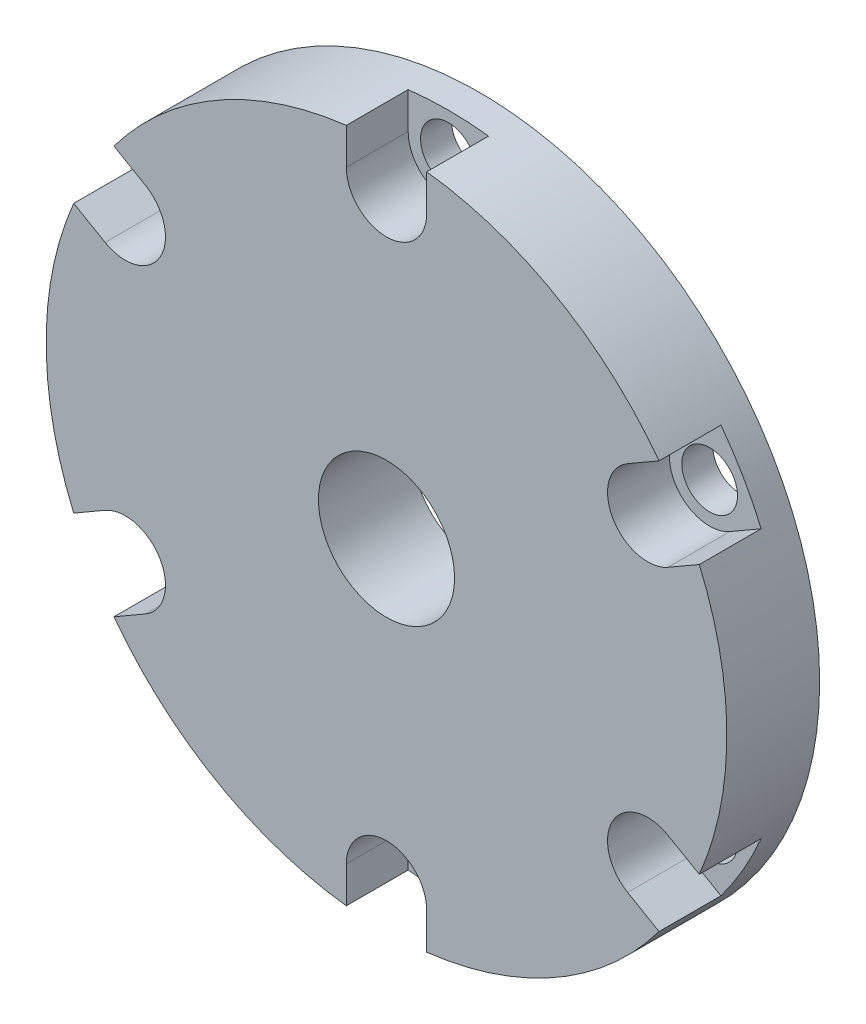
from build123d import *

# Parameters (mm, degrees)
SKETCH1_R           = 110
SKETCH1_R_2         = 9
SKETCH1_R_3         = 22
BOSS_EXTRUDE1_DEPTH = 30
CUT_EXTRUDE1_DEPTH  = 20


with BuildPart() as part:
    # Sketch1 → Boss-Extrude1 (new body)
    with BuildSketch(Plane.XY):
        Circle(SKETCH1_R)
        with Locations((0, 97.5)):
            Circle(SKETCH1_R_2, mode=Mode.SUBTRACT)
        with Locations((84.437476869, 48.75)):
            Circle(SKETCH1_R_2, mode=Mode.SUBTRACT)
        with Locations((84.437476869, -48.75)):
            Circle(SKETCH1_R_2, mode=Mode.SUBTRACT)
        with Locations((0, -97.5)):
            Circle(SKETCH1_R_2, mode=Mode.SUBTRACT)
        with Locations((-84.437476869, -48.75)):
            Circle(SKETCH1_R_2, mode=Mode.SUBTRACT)
        with Locations((-84.437476869, 48.75)):
            Circle(SKETCH1_R_2, mode=Mode.SUBTRACT)
        Circle(SKETCH1_R_3, mode=Mode.SUBTRACT)
    extrude(amount=BOSS_EXTRUDE1_DEPTH)

    # Sketch2 → Cut-Extrude1 (cut)
    with BuildSketch(Plane.XY.offset(30)):
        with BuildLine():
            Line((-13, 97.5), (-13, 114.531439902))
            Line((-13, 114.531439902), (13, 114.531439902))
            Line((13, 114.531439902), (13, 97.5))
            ThreePointArc((13, 97.5), (0, 84.5), (-13, 97.5))
        make_face()
        with BuildLine():
            Line((105.687136487, 46.007389702), (90.937476869, 37.491669751))
            ThreePointArc((90.937476869, 37.491669751), (73.17914662, 42.25), (77.937476869, 60.008330249))
            Line((77.937476869, 60.008330249), (92.687136487, 68.5240502))
            Line((92.687136487, 68.5240502), (105.687136487, 46.007389702))
        make_face()
        with BuildLine():
            Line((92.687136487, -68.5240502), (77.937476869, -60.008330249))
            ThreePointArc((77.937476869, -60.008330249), (73.17914662, -42.25), (90.937476869, -37.491669751))
            Line((90.937476869, -37.491669751), (105.687136487, -46.007389702))
            Line((105.687136487, -46.007389702), (92.687136487, -68.5240502))
        make_face()
        with BuildLine():
            Line((-13, -114.531439902), (-13, -97.5))
            ThreePointArc((-13, -97.5), (0, -84.5), (13, -97.5))
            Line((13, -97.5), (13, -114.531439902))
            Line((13, -114.531439902), (-13, -114.531439902))
        make_face()
        with BuildLine():
            Line((-105.687136487, -46.007389702), (-90.937476869, -37.491669751))
            ThreePointArc((-90.937476869, -37.491669751), (-73.17914662, -42.25), (-77.937476869, -60.008330249))
            Line((-77.937476869, -60.008330249), (-92.687136487, -68.5240502))
            Line((-92.687136487, -68.5240502), (-105.687136487, -46.007389702))
        make_face()
        with BuildLine():
            Line((-92.687136487, 68.5240502), (-77.937476869, 60.008330249))
            ThreePointArc((-77.937476869, 60.008330249), (-73.17914662, 42.25), (-90.937476869, 37.491669751))
            Line((-90.937476869, 37.491669751), (-105.687136487, 46.007389702))
            Line((-105.687136487, 46.007389702), (-92.687136487, 68.5240502))
        make_face()
    extrude(amount=-CUT_EXTRUDE1_DEPTH, mode=Mode.SUBTRACT)


solid = part.part
